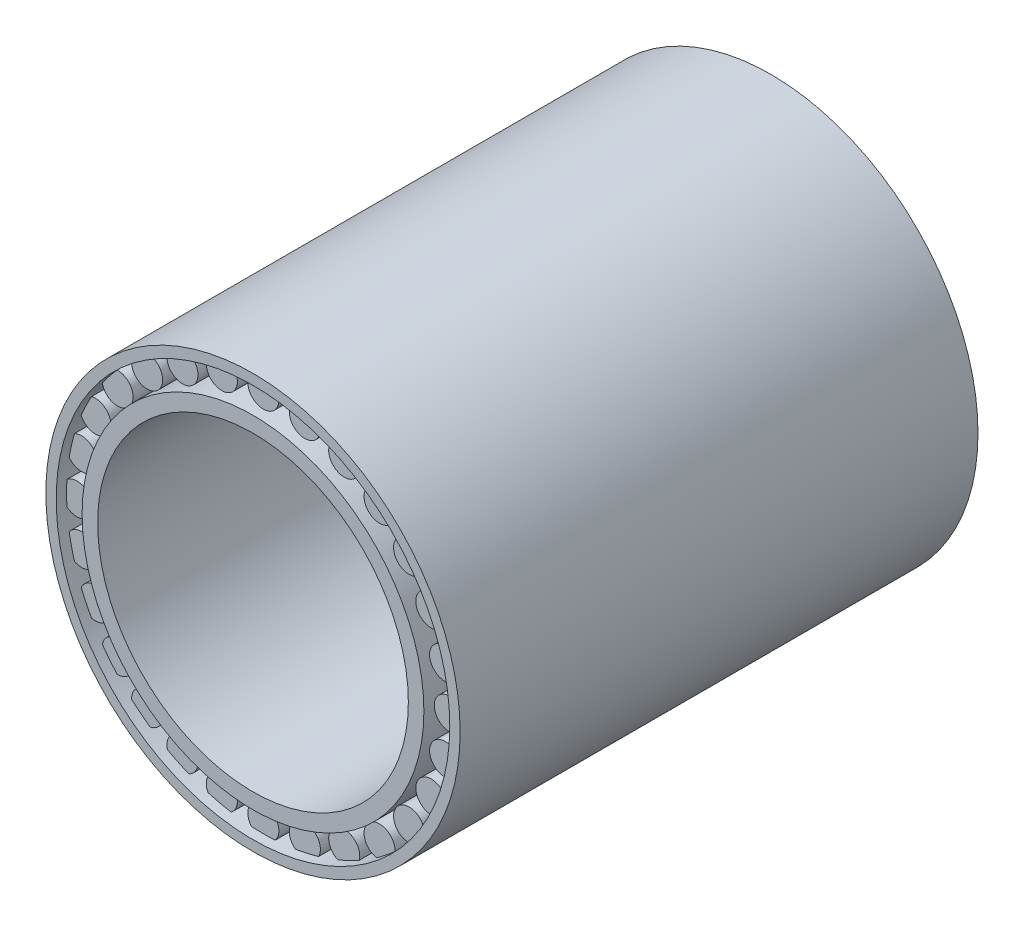
from build123d import *

# Parameters (mm, degrees)
SKETCH1_R              = 16.5
SKETCH1_R_2            = 15
BOSS_EXTRUDE1_DEPTH    = 50
BOSS_EXTRUDE2_START    = -1
SKETCH2_R              = 1.5
BOSS_EXTRUDE2_DEPTH    = 48
BOSS_EXTRUDE2_2_DEPTH  = 48
BOSS_EXTRUDE2_3_DEPTH  = 48
BOSS_EXTRUDE2_4_DEPTH  = 48
BOSS_EXTRUDE2_5_DEPTH  = 48
BOSS_EXTRUDE2_6_DEPTH  = 48
BOSS_EXTRUDE2_7_DEPTH  = 48
BOSS_EXTRUDE2_8_DEPTH  = 48
BOSS_EXTRUDE2_9_DEPTH  = 48
BOSS_EXTRUDE2_10_DEPTH = 48
BOSS_EXTRUDE2_11_DEPTH = 48
BOSS_EXTRUDE2_12_DEPTH = 48
BOSS_EXTRUDE2_13_DEPTH = 48
BOSS_EXTRUDE2_14_DEPTH = 48
BOSS_EXTRUDE2_15_DEPTH = 48
BOSS_EXTRUDE2_16_DEPTH = 48
BOSS_EXTRUDE2_17_DEPTH = 48
BOSS_EXTRUDE2_18_DEPTH = 48
BOSS_EXTRUDE2_19_DEPTH = 48
BOSS_EXTRUDE2_20_DEPTH = 48
BOSS_EXTRUDE2_21_DEPTH = 48
BOSS_EXTRUDE2_22_DEPTH = 48
BOSS_EXTRUDE2_23_DEPTH = 48
BOSS_EXTRUDE2_24_DEPTH = 48
BOSS_EXTRUDE2_25_DEPTH = 48
BOSS_EXTRUDE2_26_DEPTH = 48
BOSS_EXTRUDE2_27_DEPTH = 48
BOSS_EXTRUDE2_28_DEPTH = 48
SKETCH3_R              = 20
SKETCH3_R_2            = 19
BOSS_EXTRUDE3_DEPTH    = 50


with BuildPart() as part:
    # Sketch1 → Boss-Extrude1 (new body)
    with BuildSketch(Plane.XY):
        Circle(SKETCH1_R)
        Circle(SKETCH1_R_2, mode=Mode.SUBTRACT)
    extrude(amount=BOSS_EXTRUDE1_DEPTH)


with BuildPart() as body_2:
    # Sketch2 → Boss-Extrude2 (new body)
    with BuildSketch(Plane.XY.offset(50).offset(BOSS_EXTRUDE2_START)):
        with Locations((0, 18)):
            Circle(SKETCH2_R)
    extrude(amount=-BOSS_EXTRUDE2_DEPTH)



with BuildPart() as body_3:
    # Sketch2 → Boss-Extrude2 2 (new body)
    with BuildSketch(Plane.XY.offset(50).offset(BOSS_EXTRUDE2_START)):
        with Locations((4.005376811, 17.548702419)):
            Circle(SKETCH2_R)
    extrude(amount=-BOSS_EXTRUDE2_2_DEPTH)


with BuildPart() as body_4:
    # Sketch2 → Boss-Extrude2 3 (new body)
    with BuildSketch(Plane.XY.offset(50).offset(BOSS_EXTRUDE2_START)):
        with Locations((7.809907304, 16.217439622)):
            Circle(SKETCH2_R)
    extrude(amount=-BOSS_EXTRUDE2_3_DEPTH)


with BuildPart() as body_5:
    # Sketch2 → Boss-Extrude2 4 (new body)
    with BuildSketch(Plane.XY.offset(50).offset(BOSS_EXTRUDE2_START)):
        with Locations((11.222816433, 14.072966684)):
            Circle(SKETCH2_R)
    extrude(amount=-BOSS_EXTRUDE2_4_DEPTH)


with BuildPart() as body_6:
    # Sketch2 → Boss-Extrude2 5 (new body)
    with BuildSketch(Plane.XY.offset(50).offset(BOSS_EXTRUDE2_START)):
        with Locations((14.072966684, 11.222816433)):
            Circle(SKETCH2_R)
    extrude(amount=-BOSS_EXTRUDE2_5_DEPTH)


with BuildPart() as body_7:
    # Sketch2 → Boss-Extrude2 6 (new body)
    with BuildSketch(Plane.XY.offset(50).offset(BOSS_EXTRUDE2_START)):
        with Locations((16.217439622, 7.809907304)):
            Circle(SKETCH2_R)
    extrude(amount=-BOSS_EXTRUDE2_6_DEPTH)


with BuildPart() as body_8:
    # Sketch2 → Boss-Extrude2 7 (new body)
    with BuildSketch(Plane.XY.offset(50).offset(BOSS_EXTRUDE2_START)):
        with Locations((17.548702419, 4.005376811)):
            Circle(SKETCH2_R)
    extrude(amount=-BOSS_EXTRUDE2_7_DEPTH)


with BuildPart() as body_9:
    # Sketch2 → Boss-Extrude2 8 (new body)
    with BuildSketch(Plane.XY.offset(50).offset(BOSS_EXTRUDE2_START)):
        with Locations((18, 0)):
            Circle(SKETCH2_R)
    extrude(amount=-BOSS_EXTRUDE2_8_DEPTH)


with BuildPart() as body_10:
    # Sketch2 → Boss-Extrude2 9 (new body)
    with BuildSketch(Plane.XY.offset(50).offset(BOSS_EXTRUDE2_START)):
        with Locations((17.548702419, -4.005376811)):
            Circle(SKETCH2_R)
    extrude(amount=-BOSS_EXTRUDE2_9_DEPTH)


with BuildPart() as body_11:
    # Sketch2 → Boss-Extrude2 10 (new body)
    with BuildSketch(Plane.XY.offset(50).offset(BOSS_EXTRUDE2_START)):
        with Locations((16.217439622, -7.809907304)):
            Circle(SKETCH2_R)
    extrude(amount=-BOSS_EXTRUDE2_10_DEPTH)


with BuildPart() as body_12:
    # Sketch2 → Boss-Extrude2 11 (new body)
    with BuildSketch(Plane.XY.offset(50).offset(BOSS_EXTRUDE2_START)):
        with Locations((14.072966684, -11.222816433)):
            Circle(SKETCH2_R)
    extrude(amount=-BOSS_EXTRUDE2_11_DEPTH)


with BuildPart() as body_13:
    # Sketch2 → Boss-Extrude2 12 (new body)
    with BuildSketch(Plane.XY.offset(50).offset(BOSS_EXTRUDE2_START)):
        with Locations((11.222816433, -14.072966684)):
            Circle(SKETCH2_R)
    extrude(amount=-BOSS_EXTRUDE2_12_DEPTH)


with BuildPart() as body_14:
    # Sketch2 → Boss-Extrude2 13 (new body)
    with BuildSketch(Plane.XY.offset(50).offset(BOSS_EXTRUDE2_START)):
        with Locations((7.809907304, -16.217439622)):
            Circle(SKETCH2_R)
    extrude(amount=-BOSS_EXTRUDE2_13_DEPTH)


with BuildPart() as body_15:
    # Sketch2 → Boss-Extrude2 14 (new body)
    with BuildSketch(Plane.XY.offset(50).offset(BOSS_EXTRUDE2_START)):
        with Locations((4.005376811, -17.548702419)):
            Circle(SKETCH2_R)
    extrude(amount=-BOSS_EXTRUDE2_14_DEPTH)


with BuildPart() as body_16:
    # Sketch2 → Boss-Extrude2 15 (new body)
    with BuildSketch(Plane.XY.offset(50).offset(BOSS_EXTRUDE2_START)):
        with Locations((0, -18)):
            Circle(SKETCH2_R)
    extrude(amount=-BOSS_EXTRUDE2_15_DEPTH)


with BuildPart() as body_17:
    # Sketch2 → Boss-Extrude2 16 (new body)
    with BuildSketch(Plane.XY.offset(50).offset(BOSS_EXTRUDE2_START)):
        with Locations((-4.005376811, -17.548702419)):
            Circle(SKETCH2_R)
    extrude(amount=-BOSS_EXTRUDE2_16_DEPTH)


with BuildPart() as body_18:
    # Sketch2 → Boss-Extrude2 17 (new body)
    with BuildSketch(Plane.XY.offset(50).offset(BOSS_EXTRUDE2_START)):
        with Locations((-7.809907304, -16.217439622)):
            Circle(SKETCH2_R)
    extrude(amount=-BOSS_EXTRUDE2_17_DEPTH)


with BuildPart() as body_19:
    # Sketch2 → Boss-Extrude2 18 (new body)
    with BuildSketch(Plane.XY.offset(50).offset(BOSS_EXTRUDE2_START)):
        with Locations((-11.222816433, -14.072966684)):
            Circle(SKETCH2_R)
    extrude(amount=-BOSS_EXTRUDE2_18_DEPTH)


with BuildPart() as body_20:
    # Sketch2 → Boss-Extrude2 19 (new body)
    with BuildSketch(Plane.XY.offset(50).offset(BOSS_EXTRUDE2_START)):
        with Locations((-14.072966684, -11.222816433)):
            Circle(SKETCH2_R)
    extrude(amount=-BOSS_EXTRUDE2_19_DEPTH)


with BuildPart() as body_21:
    # Sketch2 → Boss-Extrude2 20 (new body)
    with BuildSketch(Plane.XY.offset(50).offset(BOSS_EXTRUDE2_START)):
        with Locations((-16.217439622, -7.809907304)):
            Circle(SKETCH2_R)
    extrude(amount=-BOSS_EXTRUDE2_20_DEPTH)


with BuildPart() as body_22:
    # Sketch2 → Boss-Extrude2 21 (new body)
    with BuildSketch(Plane.XY.offset(50).offset(BOSS_EXTRUDE2_START)):
        with Locations((-17.548702419, -4.005376811)):
            Circle(SKETCH2_R)
    extrude(amount=-BOSS_EXTRUDE2_21_DEPTH)


with BuildPart() as body_23:
    # Sketch2 → Boss-Extrude2 22 (new body)
    with BuildSketch(Plane.XY.offset(50).offset(BOSS_EXTRUDE2_START)):
        with Locations((-18, 0)):
            Circle(SKETCH2_R)
    extrude(amount=-BOSS_EXTRUDE2_22_DEPTH)


with BuildPart() as body_24:
    # Sketch2 → Boss-Extrude2 23 (new body)
    with BuildSketch(Plane.XY.offset(50).offset(BOSS_EXTRUDE2_START)):
        with Locations((-17.548702419, 4.005376811)):
            Circle(SKETCH2_R)
    extrude(amount=-BOSS_EXTRUDE2_23_DEPTH)


with BuildPart() as body_25:
    # Sketch2 → Boss-Extrude2 24 (new body)
    with BuildSketch(Plane.XY.offset(50).offset(BOSS_EXTRUDE2_START)):
        with Locations((-16.217439622, 7.809907304)):
            Circle(SKETCH2_R)
    extrude(amount=-BOSS_EXTRUDE2_24_DEPTH)


with BuildPart() as body_26:
    # Sketch2 → Boss-Extrude2 25 (new body)
    with BuildSketch(Plane.XY.offset(50).offset(BOSS_EXTRUDE2_START)):
        with Locations((-14.072966684, 11.222816433)):
            Circle(SKETCH2_R)
    extrude(amount=-BOSS_EXTRUDE2_25_DEPTH)


with BuildPart() as body_27:
    # Sketch2 → Boss-Extrude2 26 (new body)
    with BuildSketch(Plane.XY.offset(50).offset(BOSS_EXTRUDE2_START)):
        with Locations((-11.222816433, 14.072966684)):
            Circle(SKETCH2_R)
    extrude(amount=-BOSS_EXTRUDE2_26_DEPTH)


with BuildPart() as body_28:
    # Sketch2 → Boss-Extrude2 27 (new body)
    with BuildSketch(Plane.XY.offset(50).offset(BOSS_EXTRUDE2_START)):
        with Locations((-7.809907304, 16.217439622)):
            Circle(SKETCH2_R)
    extrude(amount=-BOSS_EXTRUDE2_27_DEPTH)


with BuildPart() as body_29:
    # Sketch2 → Boss-Extrude2 28 (new body)
    with BuildSketch(Plane.XY.offset(50).offset(BOSS_EXTRUDE2_START)):
        with Locations((-4.005376811, 17.548702419)):
            Circle(SKETCH2_R)
    extrude(amount=-BOSS_EXTRUDE2_28_DEPTH)


with BuildPart() as body_2_1:
    add(body_2.part)

    add(body_3.part)  # Boss-Extrude3 merges body 3

    add(body_4.part)  # Boss-Extrude3 merges body 4

    add(body_5.part)  # Boss-Extrude3 merges body 5

    add(body_6.part)  # Boss-Extrude3 merges body 6

    add(body_7.part)  # Boss-Extrude3 merges body 7

    add(body_8.part)  # Boss-Extrude3 merges body 8

    add(body_9.part)  # Boss-Extrude3 merges body 9

    add(body_10.part)  # Boss-Extrude3 merges body 10

    add(body_11.part)  # Boss-Extrude3 merges body 11

    add(body_12.part)  # Boss-Extrude3 merges body 12

    add(body_13.part)  # Boss-Extrude3 merges body 13

    add(body_14.part)  # Boss-Extrude3 merges body 14

    add(body_15.part)  # Boss-Extrude3 merges body 15

    add(body_16.part)  # Boss-Extrude3 merges body 16

    add(body_17.part)  # Boss-Extrude3 merges body 17

    add(body_18.part)  # Boss-Extrude3 merges body 18

    add(body_19.part)  # Boss-Extrude3 merges body 19

    add(body_20.part)  # Boss-Extrude3 merges body 20

    add(body_21.part)  # Boss-Extrude3 merges body 21

    add(body_22.part)  # Boss-Extrude3 merges body 22

    add(body_23.part)  # Boss-Extrude3 merges body 23

    add(body_24.part)  # Boss-Extrude3 merges body 24

    add(body_25.part)  # Boss-Extrude3 merges body 25

    add(body_26.part)  # Boss-Extrude3 merges body 26

    add(body_27.part)  # Boss-Extrude3 merges body 27

    add(body_28.part)  # Boss-Extrude3 merges body 28

    add(body_29.part)  # Boss-Extrude3 merges body 29
    # Sketch3 → Boss-Extrude3 (add)
    with BuildSketch(Plane.XY.offset(50)):
        Circle(SKETCH3_R)
        Circle(SKETCH3_R_2, mode=Mode.SUBTRACT)
    extrude(amount=-BOSS_EXTRUDE3_DEPTH)


solid = Compound([part.part, body_2_1.part])
